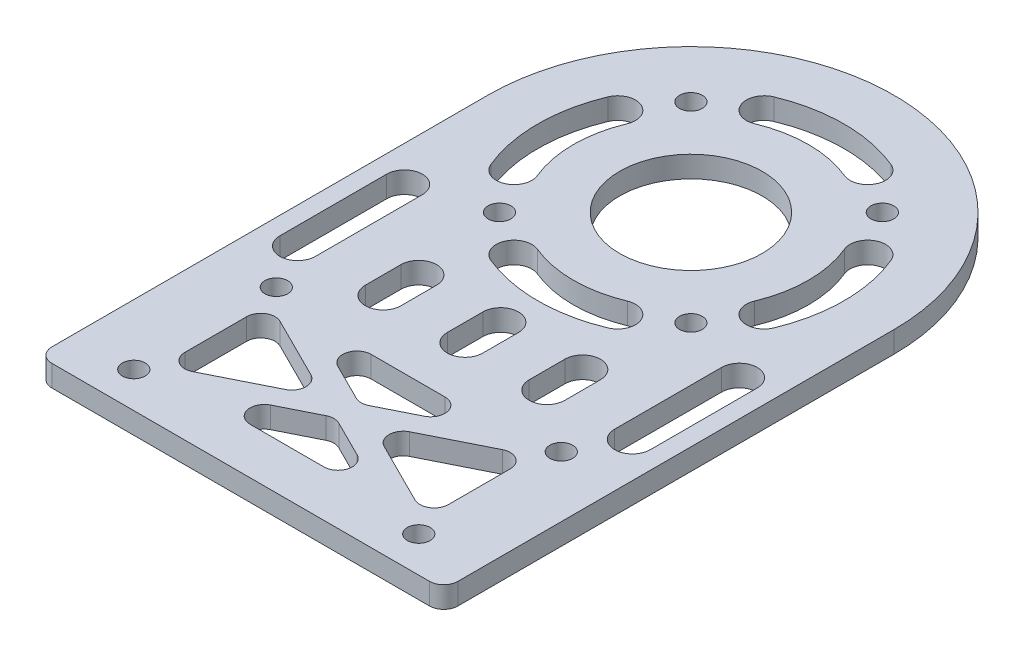
from build123d import *

# Parameters (mm, degrees)
SKETCH_1_R          = 1.6
SKETCH_1_R_2        = 10
EXTRUDE_1_DEPTH     = 3
CUT_EXTRUDE_1_DEPTH = 3
FILLET_1_R          = 2


with BuildPart() as part:
    # 草图1 → 凸台-拉伸1 (new body)
    with BuildSketch(Plane(origin=(0, 0, 0), x_dir=(1, 0, 0), z_dir=(0, 1, 0))):
        with BuildLine():
            Line((-28.5, 0), (-28.5, -63.2))
            Line((-28.5, -63.2), (28.5, -63.2))
            Line((28.5, -63.2), (28.5, 0))
            ThreePointArc((28.5, 0), (0, 28.5), (-28.5, 0))
        make_face()
        with Locations(Location((-20, -38.2, 0), (0, 0, 270))):
            Circle(SKETCH_1_R, mode=Mode.SUBTRACT)
        with Locations(Location((20, -38.2, 0), (0, 0, 270))):
            Circle(SKETCH_1_R, mode=Mode.SUBTRACT)
        with Locations(Location((20, -58.2, 0), (0, 0, 270))):
            Circle(SKETCH_1_R, mode=Mode.SUBTRACT)
        with Locations(Location((-20, -58.2, 0), (0, 0, 270))):
            Circle(SKETCH_1_R, mode=Mode.SUBTRACT)
        with Locations(Location((0, 0, 0), (0, 0, 270))):
            Circle(SKETCH_1_R_2, mode=Mode.SUBTRACT)
        with Locations(Location((-13.435028843, 13.435028843, 0), (0, 0, 270))):
            Circle(SKETCH_1_R, mode=Mode.SUBTRACT)
        with Locations(Location((13.435028843, 13.435028843, 0), (0, 0, 270))):
            Circle(SKETCH_1_R, mode=Mode.SUBTRACT)
        with Locations(Location((13.435028843, -13.435028843, 0), (0, 0, 270))):
            Circle(SKETCH_1_R, mode=Mode.SUBTRACT)
        with Locations(Location((-13.435028843, -13.435028843, 0), (0, 0, 270))):
            Circle(SKETCH_1_R, mode=Mode.SUBTRACT)
    extrude(amount=EXTRUDE_1_DEPTH)

    # 草图2 → 切除-拉伸1 (cut)
    with BuildSketch(Plane(origin=(0, 3, 0), x_dir=(1, 0, 0), z_dir=(0, 1, 0))):
        Polygon((-18.5, -40.627050983), (-18.5, -55.772949017), (-3.354101966, -48.2), align=None)
        Polygon((13.645898034, -39.7), (-13.645898034, -39.7), (0, -46.522949017), align=None)
        Polygon((3.354101966, -48.2), (18.5, -55.772949017), (18.5, -40.627050983), align=None)
        Polygon((0, -49.877050983), (-13.645898034, -56.7), (13.645898034, -56.7), align=None)
        with BuildLine():
            Line((-2.5, -26.7), (-2.5, -31.7))
            ThreePointArc((-2.5, -31.7), (0, -34.2), (2.5, -31.7))
            Line((2.5, -31.7), (2.5, -26.7))
            ThreePointArc((2.5, -26.7), (0, -24.2), (-2.5, -26.7))
        make_face()
        with BuildLine():
            ThreePointArc((14, -31.7), (11.5, -34.2), (9, -31.7))
            Line((9, -31.7), (9, -26.7))
            ThreePointArc((9, -26.7), (11.5, -24.2), (14, -26.7))
            Line((14, -26.7), (14, -31.7))
        make_face()
        with BuildLine():
            ThreePointArc((26, -31.7), (23.5, -34.2), (21, -31.7))
            Line((21, -31.7), (21, -16.7))
            ThreePointArc((21, -16.7), (23.5, -14.2), (26, -16.7))
            Line((26, -16.7), (26, -31.7))
        make_face()
        with BuildLine():
            ThreePointArc((-8.227693796, -19.863409949), (0, -21.5), (8.227693796, -19.863409949))
            ThreePointArc((8.227693796, -19.863409949), (9.580684046, -16.597002537), (6.314276634, -15.244012286))
            ThreePointArc((6.314276634, -15.244012286), (0, -16.5), (-6.314276634, -15.244012286))
            ThreePointArc((-6.314276634, -15.244012286), (-9.580684046, -16.597002537), (-8.227693796, -19.863409949))
        make_face()
        with BuildLine():
            Line((-14, -26.7), (-14, -31.7))
            ThreePointArc((-14, -31.7), (-11.5, -34.2), (-9, -31.7))
            Line((-9, -31.7), (-9, -26.7))
            ThreePointArc((-9, -26.7), (-11.5, -24.2), (-14, -26.7))
        make_face()
        with BuildLine():
            Line((-26, -16.7), (-26, -31.7))
            ThreePointArc((-26, -31.7), (-23.5, -34.2), (-21, -31.7))
            Line((-21, -31.7), (-21, -16.7))
            ThreePointArc((-21, -16.7), (-23.5, -14.2), (-26, -16.7))
        make_face()
        with BuildLine():
            ThreePointArc((-19.863409949, 8.227693796), (-21.5, 0), (-19.863409949, -8.227693796))
            ThreePointArc((-19.863409949, -8.227693796), (-16.597002537, -9.580684046), (-15.244012286, -6.314276634))
            ThreePointArc((-15.244012286, -6.314276634), (-16.5, 0), (-15.244012286, 6.314276634))
            ThreePointArc((-15.244012286, 6.314276634), (-16.597002537, 9.580684046), (-19.863409949, 8.227693796))
        make_face()
        with BuildLine():
            ThreePointArc((19.863409949, -8.227693796), (21.5, 0), (19.863409949, 8.227693796))
            ThreePointArc((19.863409949, 8.227693796), (16.597002537, 9.580684046), (15.244012286, 6.314276634))
            ThreePointArc((15.244012286, 6.314276634), (16.5, 0), (15.244012286, -6.314276634))
            ThreePointArc((15.244012286, -6.314276634), (16.597002537, -9.580684046), (19.863409949, -8.227693796))
        make_face()
        with BuildLine():
            ThreePointArc((8.227693796, 19.863409949), (0, 21.5), (-8.227693796, 19.863409949))
            ThreePointArc((-8.227693796, 19.863409949), (-9.580684046, 16.597002537), (-6.314276634, 15.244012286))
            ThreePointArc((-6.314276634, 15.244012286), (0, 16.5), (6.314276634, 15.244012286))
            ThreePointArc((6.314276634, 15.244012286), (9.580684046, 16.597002537), (8.227693796, 19.863409949))
        make_face()
    extrude(amount=-CUT_EXTRUDE_1_DEPTH, mode=Mode.SUBTRACT)

    # 圆角1
    fillet_1_edges = [part.edges().sort_by_distance(p)[0] for p in [
        (3.354101966, 1.5, 48.2),
        (18.5, 1.5, 40.627050983),
        (18.5, 1.5, 55.772949017),
        (-13.645898034, 1.5, 39.7),
        (13.645898034, 1.5, 39.7),
        (0, 1.5, 46.522949017),
        (-13.645898034, 1.5, 56.7),
        (0, 1.5, 49.877050983),
        (13.645898034, 1.5, 56.7),
        (-18.5, 1.5, 55.772949017),
        (-18.5, 1.5, 40.627050983),
        (-3.354101966, 1.5, 48.2),
        (28.5, 1.5, 63.2),
        (-28.5, 1.5, 63.2),
    ]]
    fillet(fillet_1_edges, radius=FILLET_1_R)


solid = part.part
